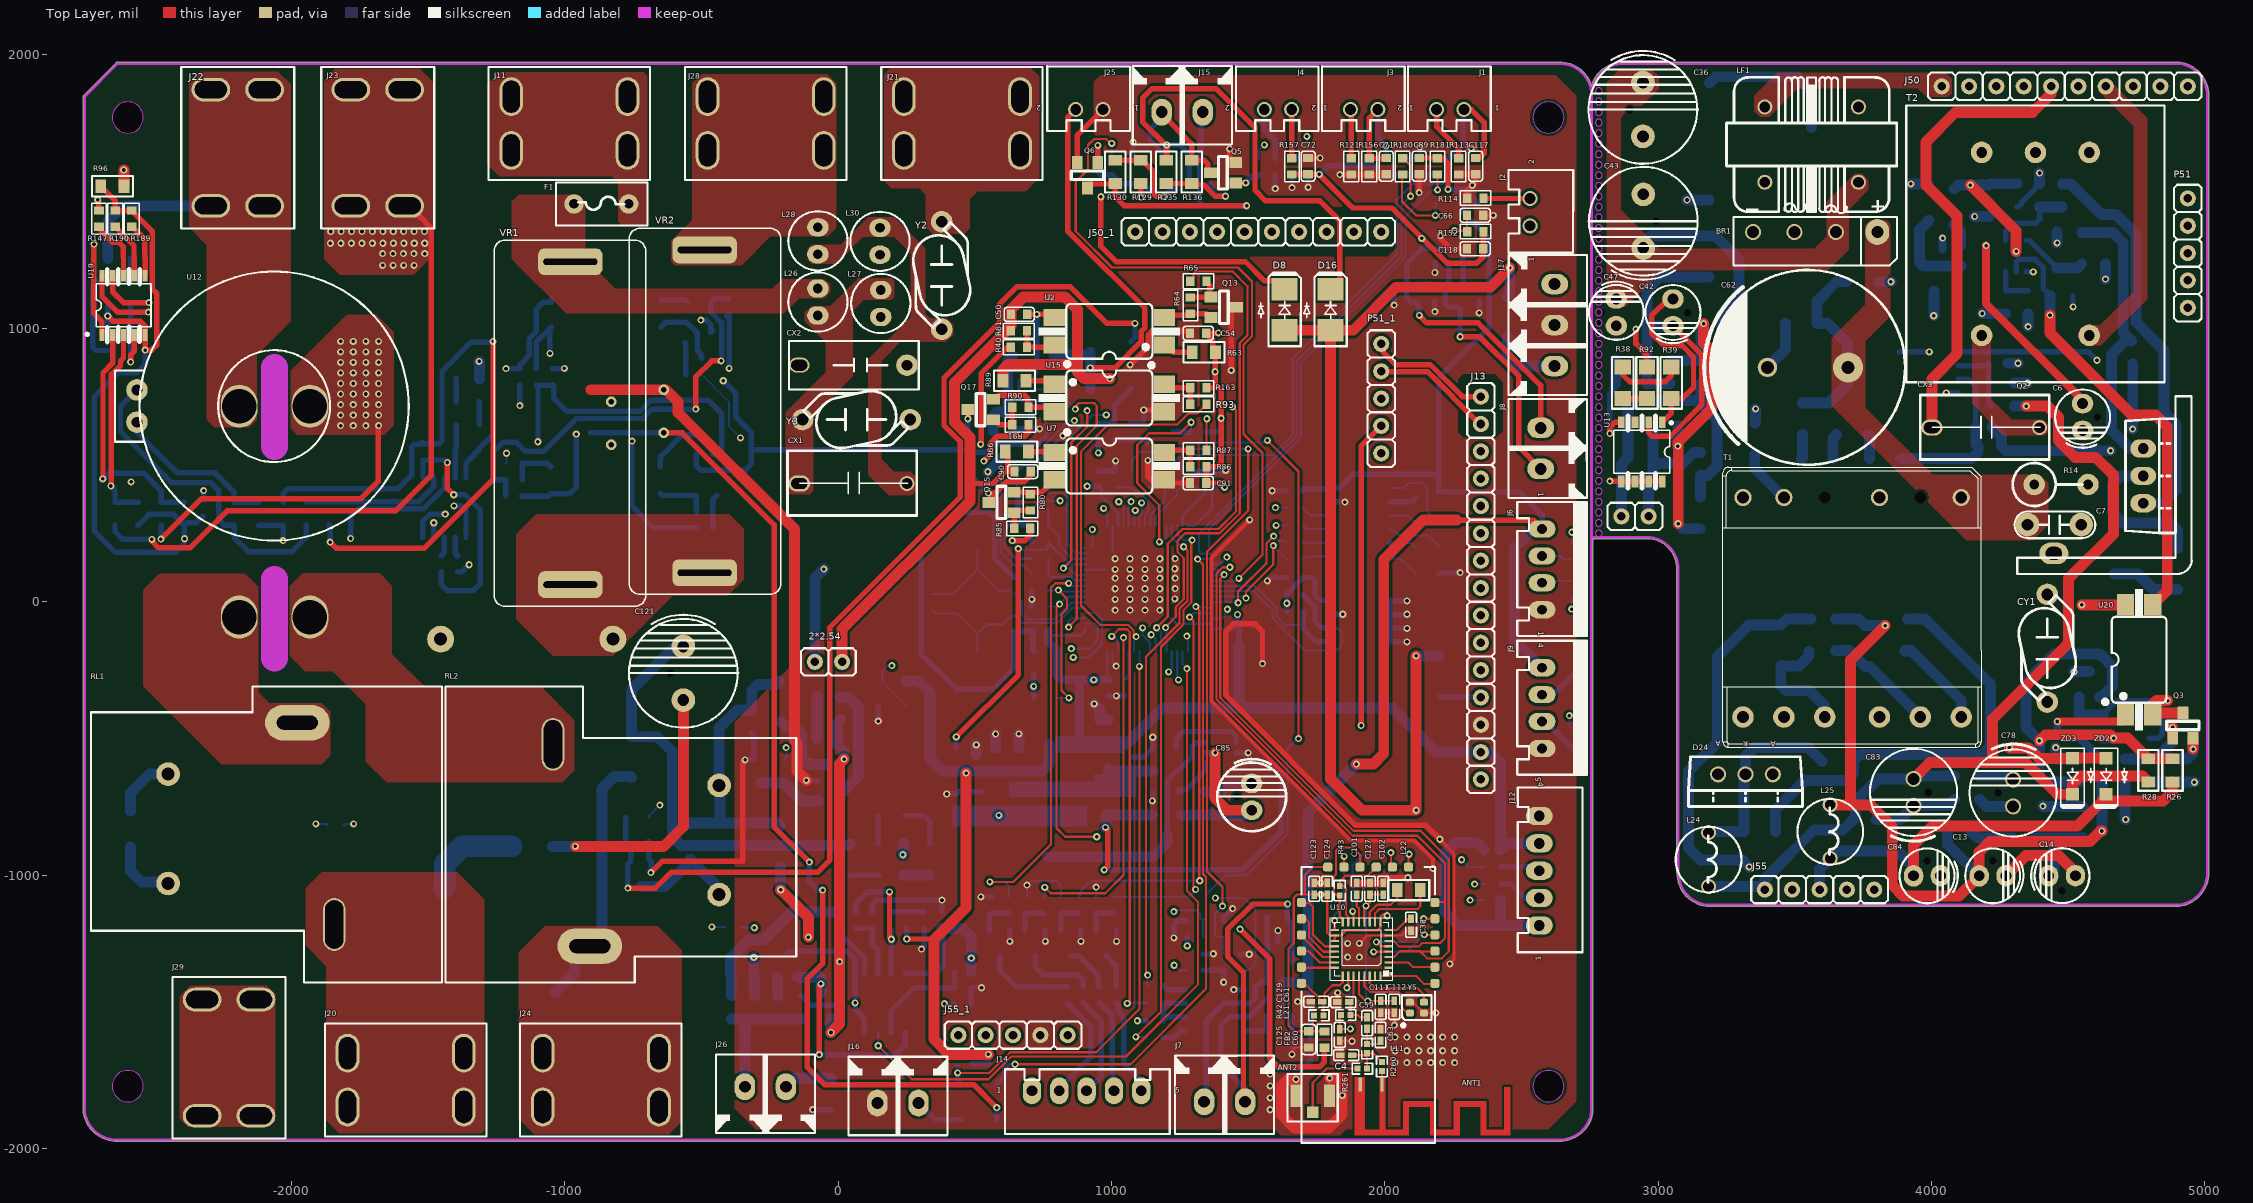
[diagram p0: Top Layer view]
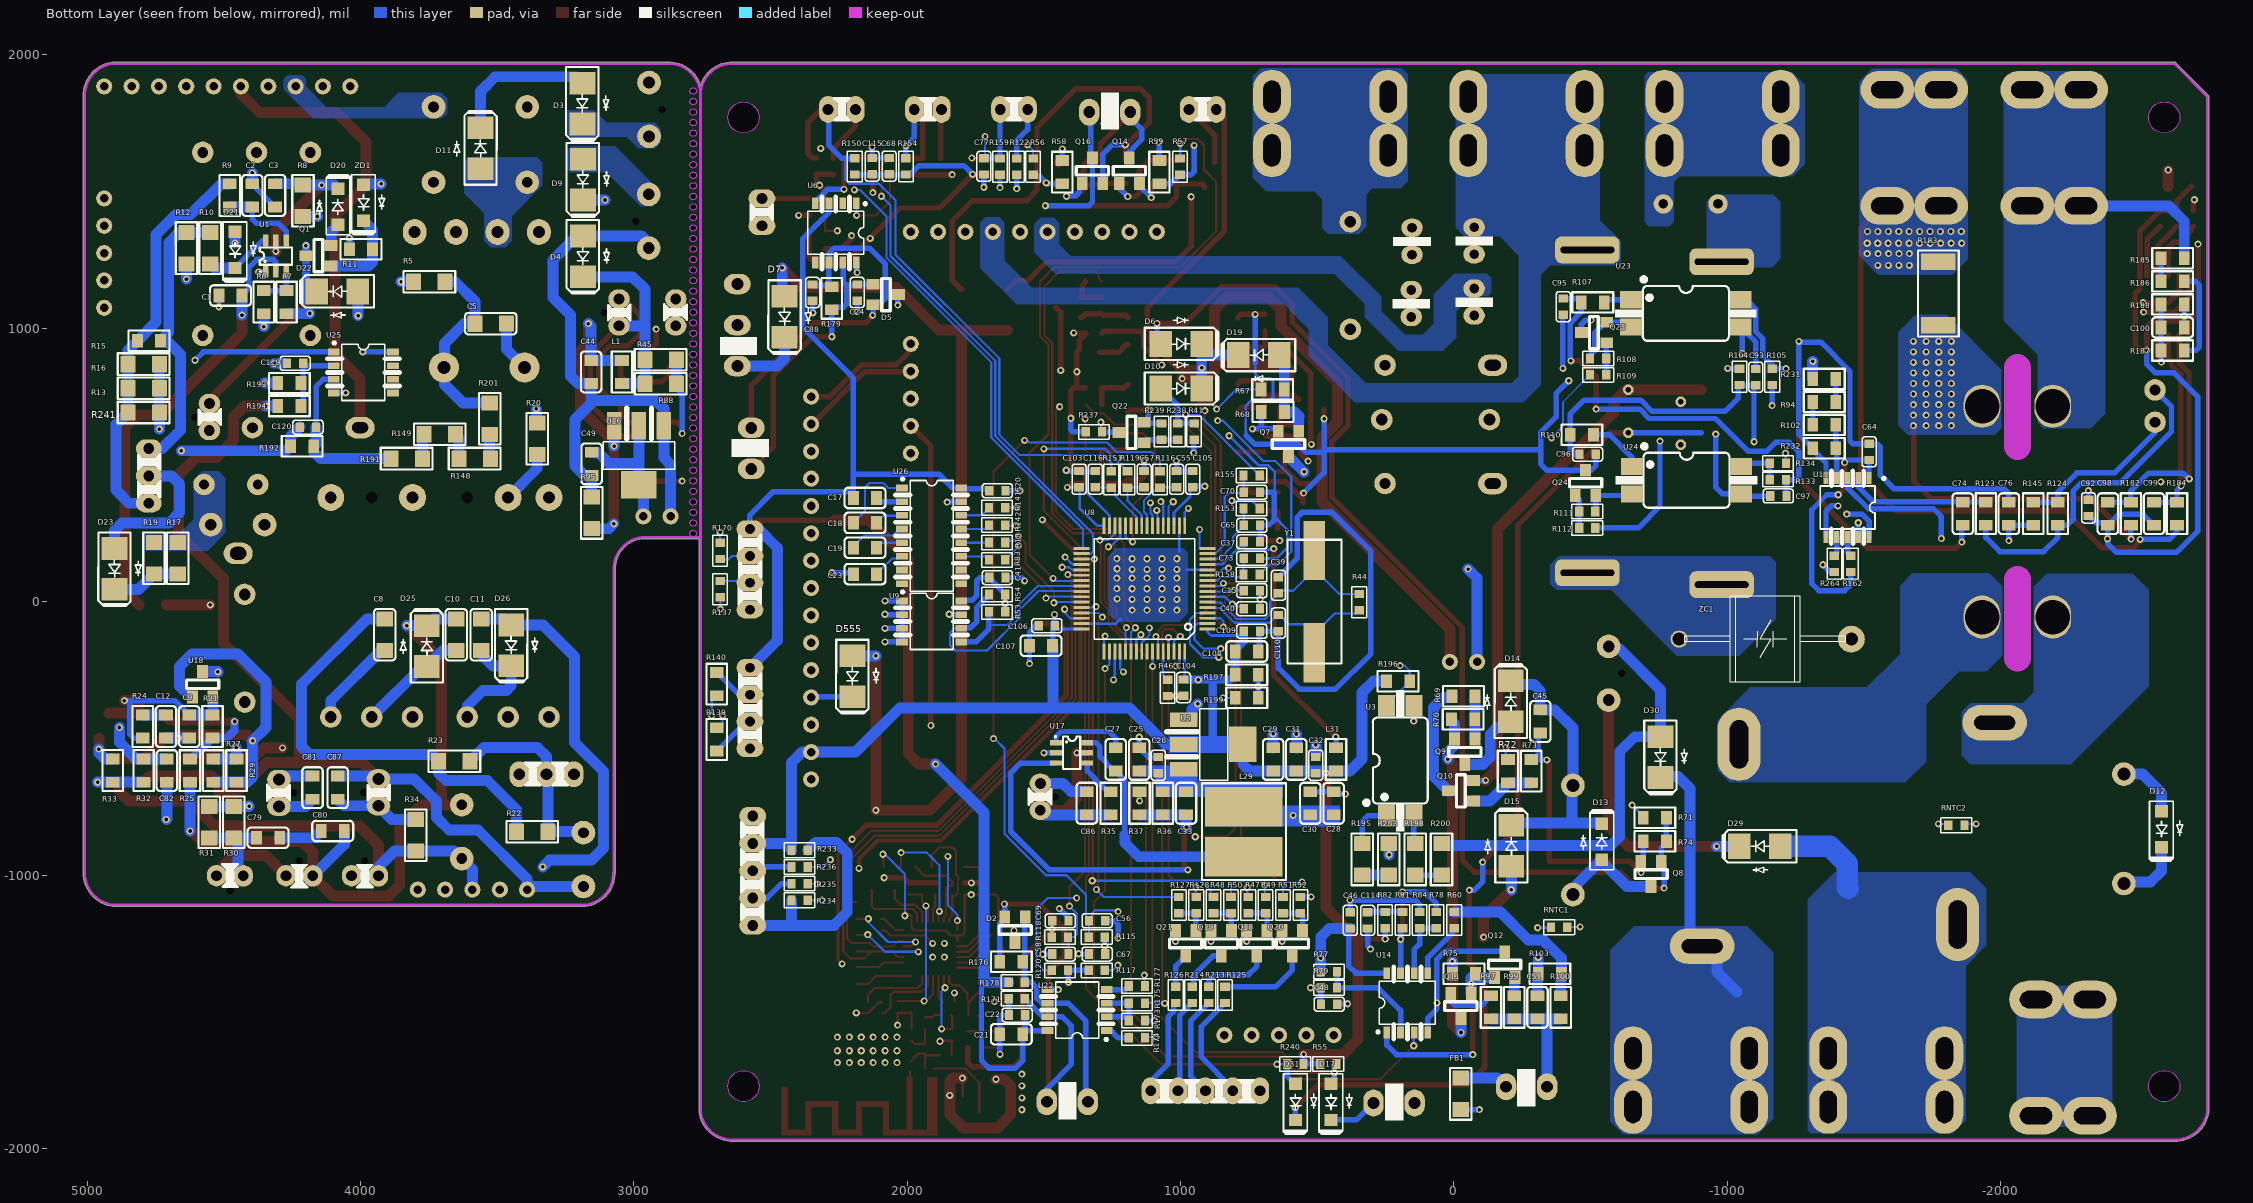
[diagram p1: Bottom Layer view, seen from below]
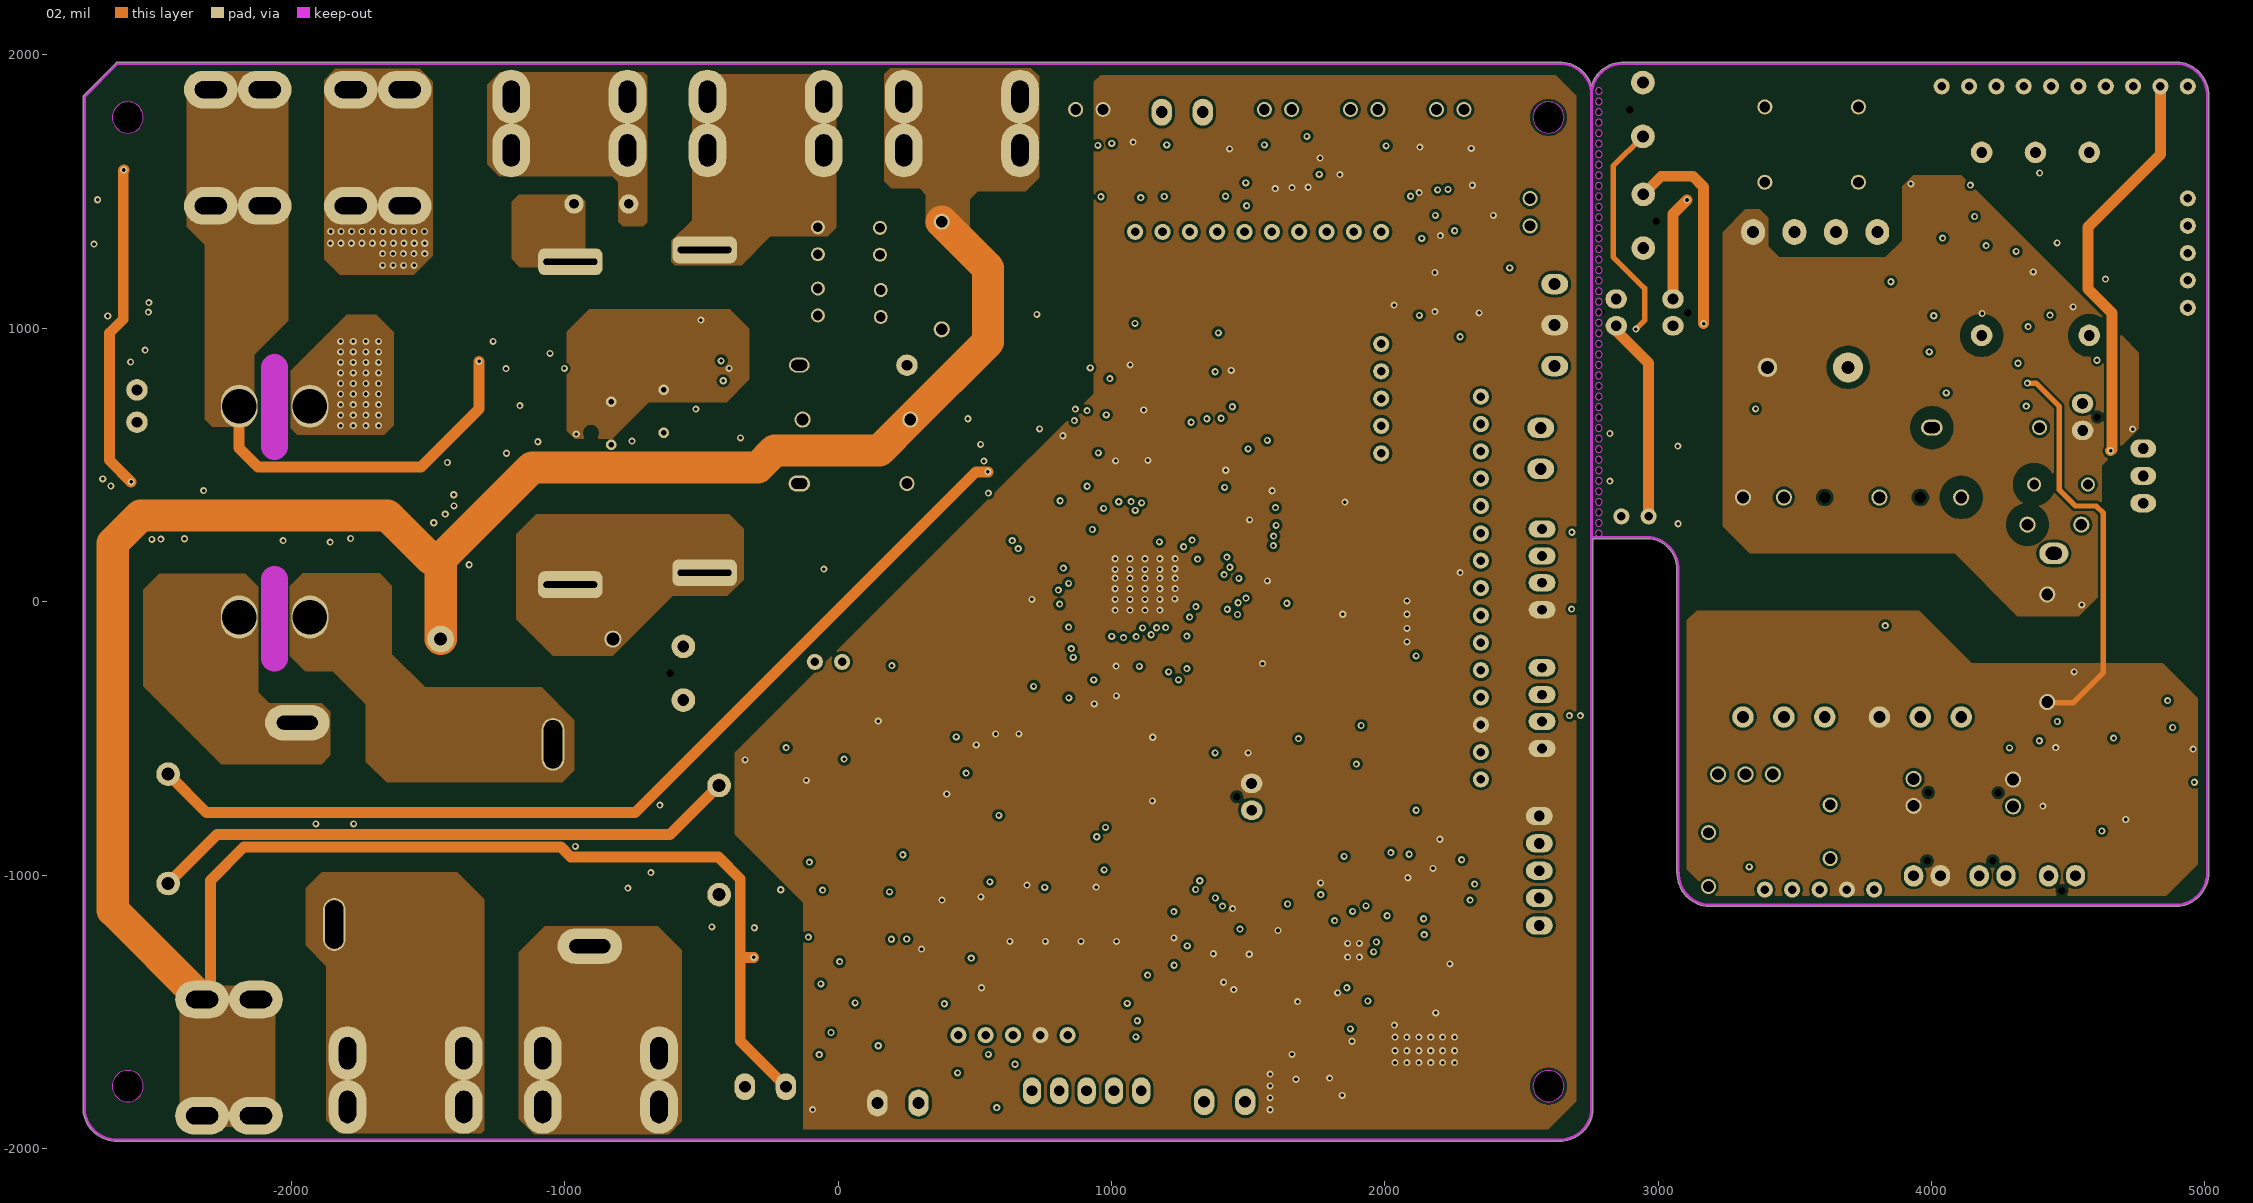
[diagram p2: 02]
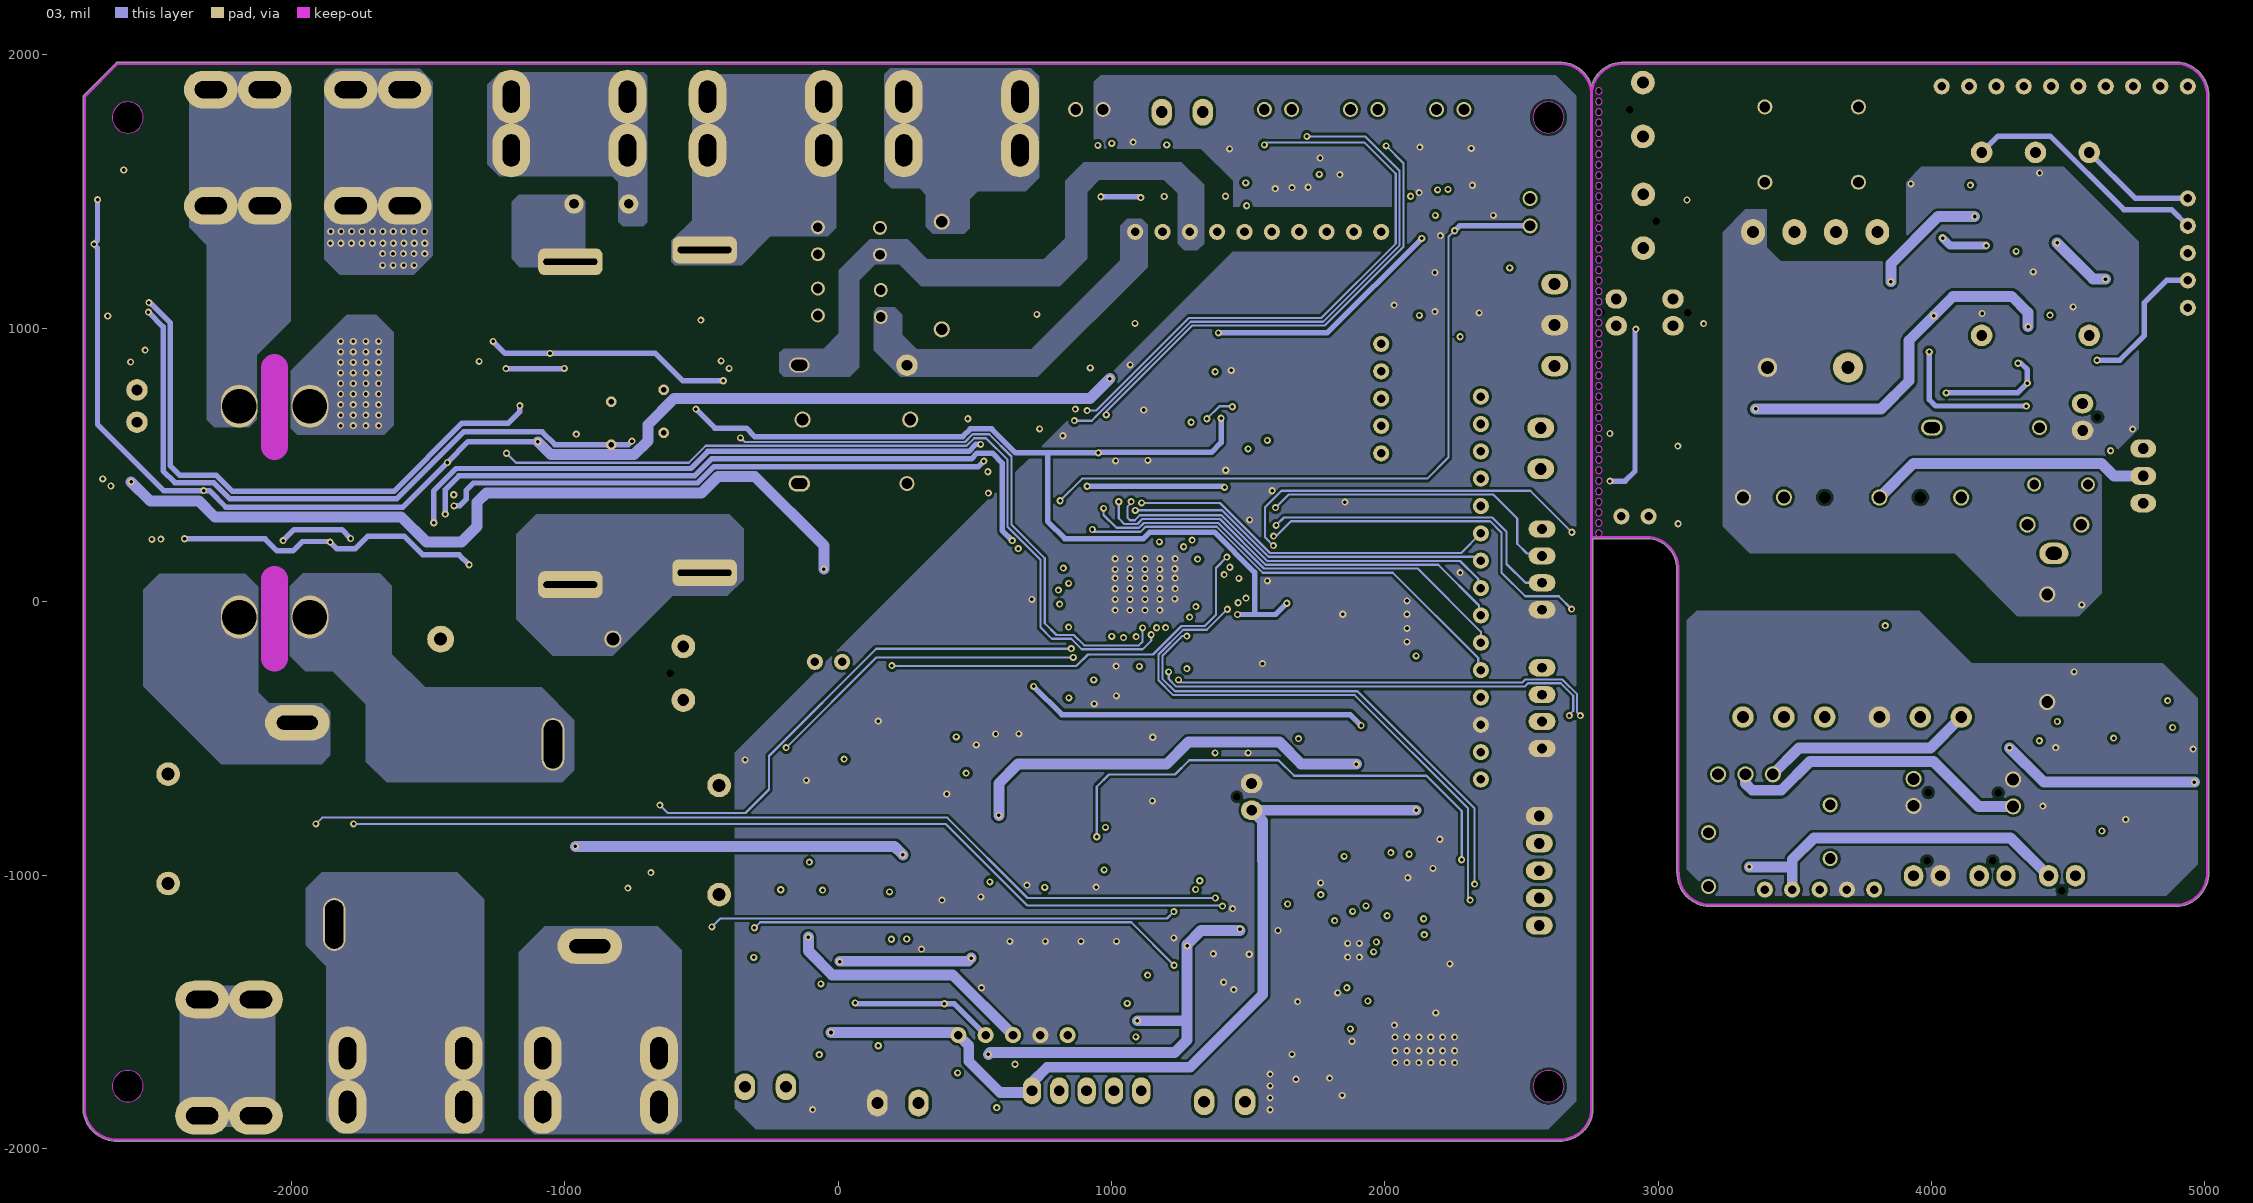
[diagram p3: 03]
# Altium PCB MISC105418.PcbDoc (part 1 of 7)
Units mil, origin at the board's own origin, x right, y up, seen from the top; angles counter-clockwise.
Board outline 7774.32 x 3947.04 mil, 4 copper layers (Top Layer, 02, 03, Bottom Layer), stack 30.635 mil thick; 459 components, 285 nets, 1258 pads, 468 vias.
Unrouted connection lines stored in the file: 23.

## Layer stack, top to bottom
Top Solder: solder mask 0.4, Solder Resist, Dk 3.5
Top Layer: signal copper 1.4
Dielectric 1: core 10, FR-4, Dk 4.2
02: signal copper 1.4173
Dielectric 6: prepreg 5, Dk 4.2
03: signal copper 1.4173
Dielectric 5: core 10, Dk 4.2
Bottom Layer: signal copper 1.4
Bottom Solder: solder mask 0.4, Solder Resist, Dk 3.5

## Board outline
-2760.88,-1866.88 ccw(c-2638.86,-1850.39) -2638.06,-1973.52 ccw(c-2637.91,-1968.5) -2637.91,-1973.52 2637.09,-1973.52 ccw(c2637.09,-1968.5) 2637.42,-1973.51 ccw(c2639.05,-1850.39) 2761.06,-1866.88 ccw(c2756.09,-1866.21) 2761.11,-1866.21 2761.11,230.49 2970.75,230.49 cw(c2955.28,118.46) 3068.37,119.45 ccw(c3073.28,118.46) 3068.27,118.46 3068.27,-990.5 ccw(c3073.28,-990.5) 3068.79,-992.72 ccw(c3191.91,-992.45) 3175.42,-1114.47 ccw(c3176.09,-1109.5) 3176.09,-1114.51 4906.09,-1114.51 ccw(c4906.09,-1109.5) 4906.77,-1114.47 ccw(c4890.28,-992.45) 5013.4,-992.45 ccw(c4890.28,-992.45) 5013.39,-990.41 ccw(c5008.37,-990.5) 5013,-988.56 5013,1847.57 ccw(c5008.37,1849.5) 5013.39,1849.42 ccw(c4890.28,1851.46) 5013.4,1851.46 ccw(c4890.28,1851.46) 4906.77,1973.47 ccw(c4906.09,1968.5) 4906.09,1973.52 ccw(c4906.09,1968.5) 4906.09,1973.52 2875.09,1973.52 ccw(c2875.09,1968.5) 2874.74,1973.51 ccw(c2872.95,1850.39) 2755.91,1888.6 ccw(c2638.86,1850.39) 2638.06,1973.52 ccw(c2637.91,1968.5) 2637.91,1973.52 -2636.53,1973.52 ccw(c-2636.53,1968.5) -2640.09,1972.03 -2759.47,1851.5 ccw(c-2755.91,1847.97) -2760.92,1847.97 -2760.92,-1866.21 ccw(c-2755.91,-1866.21)
cut-out: 2541.43,1771.16 ccw(c2598.52,1771.16) 2598.52,1714.07 ccw(c2598.52,1771.16) 2655.61,1771.16 ccw(c2598.52,1771.16) 2598.52,1828.24 ccw(c2598.52,1771.16)
cut-out: 2541.43,-1772.15 ccw(c2598.52,-1772.15) 2598.52,-1829.24 ccw(c2598.52,-1772.15) 2655.61,-1772.15 ccw(c2598.52,-1772.15) 2598.52,-1715.06 ccw(c2598.52,-1772.15)
cut-out: -2655.42,-1772.15 ccw(c-2598.33,-1772.15) -2598.33,-1829.24 ccw(c-2598.33,-1772.15) -2541.24,-1772.15 ccw(c-2598.33,-1772.15) -2598.33,-1715.06 ccw(c-2598.33,-1772.15)
cut-out: -2655.42,1771.16 ccw(c-2598.33,1771.16) -2598.33,1714.07 ccw(c-2598.33,1771.16) -2541.24,1771.16 ccw(c-2598.33,1771.16) -2598.33,1828.24 ccw(c-2598.33,1771.16)
cut-out: 2782.47,1879.96 ccw(c2782.47,1867.88) 2770.39,1867.88 ccw(c2782.47,1867.88) 2782.47,1855.79 ccw(c2782.47,1867.88) 2794.55,1867.88 ccw(c2782.47,1867.88)
cut-out: 2782.47,1841.42 ccw(c2782.47,1829.34) 2770.39,1829.34 ccw(c2782.47,1829.34) 2782.47,1817.26 ccw(c2782.47,1829.34) 2794.55,1829.34 ccw(c2782.47,1829.34)
cut-out: 2782.47,1802.89 ccw(c2782.47,1790.8) 2770.39,1790.8 ccw(c2782.47,1790.8) 2782.47,1778.72 ccw(c2782.47,1790.8) 2794.55,1790.8 ccw(c2782.47,1790.8)
cut-out: 2782.47,1764.35 ccw(c2782.47,1752.27) 2770.39,1752.27 ccw(c2782.47,1752.27) 2782.47,1740.19 ccw(c2782.47,1752.27) 2794.55,1752.27 ccw(c2782.47,1752.27)
cut-out: 2782.47,1725.81 ccw(c2782.47,1713.73) 2770.39,1713.73 ccw(c2782.47,1713.73) 2782.47,1701.65 ccw(c2782.47,1713.73) 2794.55,1713.73 ccw(c2782.47,1713.73)
cut-out: 2782.47,1687.28 ccw(c2782.47,1675.19) 2770.39,1675.19 ccw(c2782.47,1675.19) 2782.47,1663.11 ccw(c2782.47,1675.19) 2794.55,1675.19 ccw(c2782.47,1675.19)
cut-out: 2782.47,1648.74 ccw(c2782.47,1636.66) 2770.39,1636.66 ccw(c2782.47,1636.66) 2782.47,1624.58 ccw(c2782.47,1636.66) 2794.55,1636.66 ccw(c2782.47,1636.66)
cut-out: 2782.47,1610.2 ccw(c2782.47,1598.12) 2770.39,1598.12 ccw(c2782.47,1598.12) 2782.47,1586.04 ccw(c2782.47,1598.12) 2794.55,1598.12 ccw(c2782.47,1598.12)
cut-out: 2782.47,1571.67 ccw(c2782.47,1559.59) 2770.39,1559.59 ccw(c2782.47,1559.59) 2782.47,1547.5 ccw(c2782.47,1559.59) 2794.55,1559.59 ccw(c2782.47,1559.59)
cut-out: 2782.47,1533.13 ccw(c2782.47,1521.05) 2770.39,1521.05 ccw(c2782.47,1521.05) 2782.47,1508.97 ccw(c2782.47,1521.05) 2794.55,1521.05 ccw(c2782.47,1521.05)
cut-out: 2782.47,1494.59 ccw(c2782.47,1482.51) 2770.39,1482.51 ccw(c2782.47,1482.51) 2782.47,1470.43 ccw(c2782.47,1482.51) 2794.55,1482.51 ccw(c2782.47,1482.51)
cut-out: 2782.47,1456.06 ccw(c2782.47,1443.98) 2770.39,1443.98 ccw(c2782.47,1443.98) 2782.47,1431.89 ccw(c2782.47,1443.98) 2794.55,1443.98 ccw(c2782.47,1443.98)
cut-out: 2782.47,1417.52 ccw(c2782.47,1405.44) 2770.39,1405.44 ccw(c2782.47,1405.44) 2782.47,1393.36 ccw(c2782.47,1405.44) 2794.55,1405.44 ccw(c2782.47,1405.44)
cut-out: 2782.47,1378.99 ccw(c2782.47,1366.9) 2770.39,1366.9 ccw(c2782.47,1366.9) 2782.47,1354.82 ccw(c2782.47,1366.9) 2794.55,1366.9 ccw(c2782.47,1366.9)
cut-out: 2782.47,1340.45 ccw(c2782.47,1328.37) 2770.39,1328.37 ccw(c2782.47,1328.37) 2782.47,1316.28 ccw(c2782.47,1328.37) 2794.55,1328.37 ccw(c2782.47,1328.37)
cut-out: 2782.47,1301.91 ccw(c2782.47,1289.83) 2770.39,1289.83 ccw(c2782.47,1289.83) 2782.47,1277.75 ccw(c2782.47,1289.83) 2794.55,1289.83 ccw(c2782.47,1289.83)
cut-out: 2782.47,1263.38 ccw(c2782.47,1251.29) 2770.39,1251.29 ccw(c2782.47,1251.29) 2782.47,1239.21 ccw(c2782.47,1251.29) 2794.55,1251.29 ccw(c2782.47,1251.29)
cut-out: 2782.47,1224.84 ccw(c2782.47,1212.76) 2770.39,1212.76 ccw(c2782.47,1212.76) 2782.47,1200.67 ccw(c2782.47,1212.76) 2794.55,1212.76 ccw(c2782.47,1212.76)
cut-out: 2782.47,1200.67 ccw(c2782.47,1212.76) 2794.55,1212.76 ccw(c2782.47,1212.76) 2782.47,1224.84 ccw(c2782.47,1212.76) 2770.39,1212.76 ccw(c2782.47,1212.76)
cut-out: 2782.47,1162.14 ccw(c2782.47,1174.22) 2794.55,1174.22 ccw(c2782.47,1174.22) 2782.47,1186.3 ccw(c2782.47,1174.22) 2770.39,1174.22 ccw(c2782.47,1174.22)
cut-out: 2782.47,1123.6 ccw(c2782.47,1135.68) 2794.55,1135.68 ccw(c2782.47,1135.68) 2782.47,1147.77 ccw(c2782.47,1135.68) 2770.39,1135.68 ccw(c2782.47,1135.68)
cut-out: 2782.47,1085.06 ccw(c2782.47,1097.15) 2794.55,1097.15 ccw(c2782.47,1097.15) 2782.47,1109.23 ccw(c2782.47,1097.15) 2770.39,1097.15 ccw(c2782.47,1097.15)
cut-out: 2782.47,1046.53 ccw(c2782.47,1058.61) 2794.55,1058.61 ccw(c2782.47,1058.61) 2782.47,1070.69 ccw(c2782.47,1058.61) 2770.39,1058.61 ccw(c2782.47,1058.61)
cut-out: 2782.47,1007.99 ccw(c2782.47,1020.07) 2794.55,1020.07 ccw(c2782.47,1020.07) 2782.47,1032.16 ccw(c2782.47,1020.07) 2770.39,1020.07 ccw(c2782.47,1020.07)
cut-out: 2782.47,969.45 ccw(c2782.47,981.54) 2794.55,981.54 ccw(c2782.47,981.54) 2782.47,993.62 ccw(c2782.47,981.54) 2770.39,981.54 ccw(c2782.47,981.54)
cut-out: 2782.47,930.92 ccw(c2782.47,943) 2794.55,943 ccw(c2782.47,943) 2782.47,955.08 ccw(c2782.47,943) 2770.39,943 ccw(c2782.47,943)
cut-out: 2782.47,892.38 ccw(c2782.47,904.46) 2794.55,904.46 ccw(c2782.47,904.46) 2782.47,916.55 ccw(c2782.47,904.46) 2770.39,904.46 ccw(c2782.47,904.46)
cut-out: 2782.47,853.84 ccw(c2782.47,865.93) 2794.55,865.93 ccw(c2782.47,865.93) 2782.47,878.01 ccw(c2782.47,865.93) 2770.39,865.93 ccw(c2782.47,865.93)
cut-out: 2782.47,815.31 ccw(c2782.47,827.39) 2794.55,827.39 ccw(c2782.47,827.39) 2782.47,839.47 ccw(c2782.47,827.39) 2770.39,827.39 ccw(c2782.47,827.39)
cut-out: 2782.47,776.77 ccw(c2782.47,788.85) 2794.55,788.85 ccw(c2782.47,788.85) 2782.47,800.94 ccw(c2782.47,788.85) 2770.39,788.85 ccw(c2782.47,788.85)
cut-out: 2782.47,738.23 ccw(c2782.47,750.32) 2794.55,750.32 ccw(c2782.47,750.32) 2782.47,762.4 ccw(c2782.47,750.32) 2770.39,750.32 ccw(c2782.47,750.32)
cut-out: 2782.47,699.7 ccw(c2782.47,711.78) 2794.55,711.78 ccw(c2782.47,711.78) 2782.47,723.86 ccw(c2782.47,711.78) 2770.39,711.78 ccw(c2782.47,711.78)
cut-out: 2782.47,661.16 ccw(c2782.47,673.24) 2794.55,673.24 ccw(c2782.47,673.24) 2782.47,685.33 ccw(c2782.47,673.24) 2770.39,673.24 ccw(c2782.47,673.24)
cut-out: 2782.47,622.62 ccw(c2782.47,634.71) 2794.55,634.71 ccw(c2782.47,634.71) 2782.47,646.79 ccw(c2782.47,634.71) 2770.39,634.71 ccw(c2782.47,634.71)
cut-out: 2782.47,584.09 ccw(c2782.47,596.17) 2794.55,596.17 ccw(c2782.47,596.17) 2782.47,608.25 ccw(c2782.47,596.17) 2770.39,596.17 ccw(c2782.47,596.17)
cut-out: 2782.47,545.55 ccw(c2782.47,557.63) 2794.55,557.63 ccw(c2782.47,557.63) 2782.47,569.72 ccw(c2782.47,557.63) 2770.39,557.63 ccw(c2782.47,557.63)
cut-out: 2782.47,507.01 ccw(c2782.47,519.1) 2794.55,519.1 ccw(c2782.47,519.1) 2782.47,531.18 ccw(c2782.47,519.1) 2770.39,519.1 ccw(c2782.47,519.1)
cut-out: 2782.47,429.94 ccw(c2782.47,442.02) 2794.55,442.02 ccw(c2782.47,442.02) 2782.47,454.11 ccw(c2782.47,442.02) 2770.39,442.02 ccw(c2782.47,442.02)
cut-out: 2782.47,622.62 ccw(c2782.47,634.71) 2794.55,634.71 ccw(c2782.47,634.71) 2782.47,646.79 ccw(c2782.47,634.71) 2770.39,634.71 ccw(c2782.47,634.71)
cut-out: 2782.47,584.09 ccw(c2782.47,596.17) 2794.55,596.17 ccw(c2782.47,596.17) 2782.47,608.25 ccw(c2782.47,596.17) 2770.39,596.17 ccw(c2782.47,596.17)
cut-out: 2782.47,545.55 ccw(c2782.47,557.63) 2794.55,557.63 ccw(c2782.47,557.63) 2782.47,569.72 ccw(c2782.47,557.63) 2770.39,557.63 ccw(c2782.47,557.63)
cut-out: 2782.47,507.01 ccw(c2782.47,519.1) 2794.55,519.1 ccw(c2782.47,519.1) 2782.47,531.18 ccw(c2782.47,519.1) 2770.39,519.1 ccw(c2782.47,519.1)
cut-out: 2782.47,468.48 ccw(c2782.47,480.56) 2794.55,480.56 ccw(c2782.47,480.56) 2782.47,492.64 ccw(c2782.47,480.56) 2770.39,480.56 ccw(c2782.47,480.56)
cut-out: 2782.47,391.4 ccw(c2782.47,403.49) 2794.55,403.49 ccw(c2782.47,403.49) 2782.47,415.57 ccw(c2782.47,403.49) 2770.39,403.49 ccw(c2782.47,403.49)
cut-out: 2782.47,352.87 ccw(c2782.47,364.95) 2794.55,364.95 ccw(c2782.47,364.95) 2782.47,377.03 ccw(c2782.47,364.95) 2770.39,364.95 ccw(c2782.47,364.95)
cut-out: 2782.47,314.33 ccw(c2782.47,326.41) 2794.55,326.41 ccw(c2782.47,326.41) 2782.47,338.5 ccw(c2782.47,326.41) 2770.39,326.41 ccw(c2782.47,326.41)
cut-out: 2782.47,275.79 ccw(c2782.47,287.88) 2794.55,287.88 ccw(c2782.47,287.88) 2782.47,299.96 ccw(c2782.47,287.88) 2770.39,287.88 ccw(c2782.47,287.88)
cut-out: 2782.47,237.26 ccw(c2782.47,249.34) 2794.55,249.34 ccw(c2782.47,249.34) 2782.47,261.42 ccw(c2782.47,249.34) 2770.39,249.34 ccw(c2782.47,249.34)

## Design rules (kind name [scope] priority, off if disabled: settings)
Clearance [All] p1: gap=6 except(10: Arc-Fill Arc-Poly Arc-Region Track-Fill Track-Poly Track-Region SMDPad-Fill SMDPad-Poly SMDPad-Region THPad-Fill THPad-Poly THPad-Region Via-Fill Via-Poly Via-Region Fill-Fill Fill-Poly Fill-Region Poly-Poly Poly-Region Region-Region)
PlaneConnect [All] p1: planeconnectstyle=NoConnect reliefexpansion=20 reliefentries=4 reliefconductorwidth=10 reliefairgap=10
PolygonConnect [All] p1: connectstyle=Direct reliefconductorwidth=10 reliefentries=4 polygonreliefangle="90 Angle" airgapwidth=10
RoutingVias [All] p1: holewidth=13 width=26 viastyle="Through Hole" minholewidth=1 minwidth=1 maxholewidth=50 maxwidth=50
SolderMaskExpansion [All] p1: expansion=4
Width [All] p1: maxlimit=500 minlimit=6 preferedwidth=8
29 further rules are at their usual default settings.

## Classes and differential pairs
component class RELAY_V0.1: C15 C45 C46 C48 C51 C114 C119 C120 C121 D6 D10 D12 D13 D14 D15 D19 D29 D30 FB1 J20 J21 J22 J23 J24 J25 J26 J29 Q7 Q8 Q9 Q10 Q11 Q12 R60 R67 R68 R69 R70 R71 R72 R73 R74 R75 R77 R78 R79 R81 R82 R84 R97 R99 R100 R103 R148 R149 R183 R191 R192 R193 R194 R195 R196 R197 R198 R199 R200 R201 R263 RL1 RL2 U3 U14 U25
component class POWER_V0.1: BR1 C1 C2 C3 C5 C6 C7 C8 C9 C10 C11 C12 C13 C14 C25 C26 C27 C28 C29 C30 C31 C32 C33 C36 C42 C43 C44 C47 C49 C62 C78 C79 C80 C81 C82 C83 C84 C85 C86 C87 CX1 CX2 CX3 CY1 D3 D4 D7 D9 D11 D20 D21 D22 D23 D24 D25 D26 F1 J11 J17 J28 J50 J55 L1 L24 L25 L26 L27 L28 L29 L30 L31 LF1 P51 Q1 Q2 Q3 R5 R6 R7 R8 R9 R10 R11 R12 R13 R14 R15 R16 R17 R19 R20 R21 R22 R23 R24 R25 R26 R27 R28 R29 R30 R31 R32 R33 R34 R35 R36 R37 R38 R39 R45 R88 R92 R95 R241 T1 T2 U1 U5 U13 U16 U17 U18 U20 VR1 VR2 Y2 Y3 ZC1 ZD1 ZD2 ZD3
component class "MCU Controller for 7KW_V0.1": C37 C39 C40 C41 C103 C104 C105 C106 C107 C108 C109 C110 D17 D31 D555 J12 J13 J14 J16 Q18 Q19 Q20 Q21 Q22 R41 R44 R46 R47 R48 R49 R50 R51 R52 R53 R54 R55 R125 R126 R127 R128 R213 R214 R233 R234 R235 R236 R237 R238 R239 R240 U8 U9 Y1
component class ElectricLeakage-Check_V0.1: C50 C54 C64 C74 C76 C90 C91 C92 C93 C95 C96 C97 C98 C99 C100 Q13 Q15 Q17 Q23 Q24 R40 R61 R63 R64 R65 R66 R80 R85 R86 R87 R89 R90 R91 R93 R94 R96 R102 R104 R105 R107 R108 R109 R110 R111 R112 R123 R124 R133 R134 R145 R147 R162 R163 R182 R184 R185 R186 R187 R188 R189 R190 R231 R232 R264 U2 U7 U11 U12 U15 U19 U23 U24
component class Communication_V0.1: C17 C18 C19 C20 C21 C22 C23 C24 C88 C89 D2 D5 J6 J7 J8 J9 R18 R83 R137 R139 R140 R141 R142 R170 R171 R173 R174 R175 R176 R177 R178 R179 R180 R181 U6 U22 U26
component class BLE_V0.1: ANT1 ANT2 C4 C38 C59 C60 C61 C63 C101 C102 C111 C112 C123 C124 C125 C127 C129 FB2 L11 L21 L22 R42 R43 R260 R261 U10 Y5
component class ADC_V0.1: C55 C56 C57 C58 C65 C66 C67 C68 C69 C70 C71 C72 C73 C77 C115 C116 C117 C118 D8 D16 J1 J2 J3 J4 J15 Q5 Q6 Q14 Q16 R56 R57 R58 R59 R113 R114 R115 R116 R117 R118 R119 R120 R121 R122 R129 R130 R135 R136 R150 R151 R152 R153 R154 R155 R156 R157 R158 R159 RNTC1 RNTC2

## Components (designator, comment, footprint, x,y, rotation, side; value= is the part's Value field where it differs from the comment)
2*2.54 "Comment" p2-2.54 14.72,-220.24 r180 top
ANT1 "PCB onboard antenna" ATN 1949.33,-1767 r0 top
ANT2 "ANT_SMA" ATN-1 1736,-1807 r90 top
BR1 "KBJ2J" BD15.22X4.5(KBP206）RS-2 3574.21,1352 r180 top
C1 "1nF" C0805-T 4475,1120 r0 bottom
C2 "100pF" C0805-T 4395.09,1486.02 r90 bottom
C3 "0.1uF" C0805-T 4312.09,1486.02 r270 bottom
C4 "0.5pF/50V" C0402-T 1859.09,-1659.03 r180 top
C5 "10nF/1KV" C1206-T 3523,1017 r180 bottom
C6 "22uF/50V" CE5-P2.5MM-AI-DS 4552.29,675.49 r270 top
C7 "222/1KV" CC7.5-P5.0MM-AI-2.5-DS 4449.09,281.5 r180 top
C8 "102/1KV" C1206-T 3911,-120.96 r90 bottom
C9 "0.1uF" C0805-T 4626.09,-456.82 r270 bottom
C10 "n.c" C1206-T 3649.09,-120.96 r90 bottom
C11 "n.c" C1206-T 3558.09,-120.96 r90 bottom
C12 "N.C" C0805-T 4711.09,-456.82 r270 bottom
C13 "100uF/16V" CE5-P2.5MM-AI-DS 4223.09,-1002.69 r0 top
C14 "100uF/16V" CE5-P2.5MM-AI-DS 4477.09,-1002.68 r180 top
C15 "0.1uF/50V" C0603-T 738.8,40.36 r180 bottom
C17 "1uF/50V" CAP/0805 2154,379 r180 bottom
C18 "1uF/50V" CAP/0805 2154,288.12 r0 bottom
C19 "1uF/50V" CAP/0805 2154,197.52 r0 bottom
C20 "0.1uF/50V" CAP/0603 1669.91,405.7 r180 bottom
C21 "10uF/10V" C0805-T 1618.98,-1582.14 r0 bottom
C22 "0.1uF/50V" C0603-T 1597.86,-1512.14 r0 bottom
C23 "1uF/50V" CAP/0805 2154.09,100.7 r180 bottom
C24 "15pF/50V" C0603-T 2183,1130.77 r90 bottom
C25 "10uF/10V" C0805-T 1151.09,-576.97 r90 bottom
C26 "0.1uF/50V" C0603-T 1081.09,-598.09 r90 bottom
C27 "0.1uF" C0805-T 1237.09,-576.97 r270 bottom
C28 "10uF/10V" C0805-T 439.9,-737.5 r90 bottom
C29 "10uF/10V" C0805-T 661.09,-576.97 r90 bottom
C30 "10uF/10V" C0805-T 524.9,-737.5 r90 bottom
C31 "10uF/10V" C0805-T 576.09,-576.97 r90 bottom
C32 "0.1uF/50V" C0603-T 505.11,-598.09 r90 bottom
C33 "47pF" C0805-T 980.08,-737.5 r270 bottom
C36 "10uF/400V" CE10-P5.0MM-AI 2945.37,1800.82 r90 top
C37 "0.1uF/50V" C0603-T 738.8,218.65 r0 bottom
C38 "1uF/50V" C0402-T 2096,-1182 r90 top
C39 "20pF/50V" C0603-T 642,60 r270 bottom
C40 "0.1uF/50V" C0603-T 738.8,-26.07 r180 bottom
C41 "0.1uF/50V" C0603-T 1669.91,88.29 r0 bottom
C42 "10uF/50V" CE5-P2.5MM-AI 3054,1058 r270 top
C43 "100uF/25V" CE10-P5.0MM-AI 2943.98,1391.21 r270 top
C44 "1uF/25V" C0805-T 3156,840.12 r90 bottom
C45 "0.1uF/50V" C0805-T -316,-438.06 r270 bottom
C46 "0.1uF/50V" C0603-T 378.89,-1165.89 r270 bottom
C47 "100uF/16V" CE5-P2.5MM-AI 2846.39,1058 r90 top
C48 "0.1uF/50V" C0603-T 456.03,-1472.5 r0 bottom
C49 "1uF/25V/0805" C0805-T 3154,504 r90 bottom
C50 "0.1uF/50V" C0603-T 662.34,1050.81 r180 top
C51 "NC" C0805-T -305.91,-1483.82 r90 bottom
C54 "0.1uF/50V" C0603-T 1316.93,981.91 r180 top
C55 "0.1uF/50V" C0603-T 1014.43,448 r90 bottom
C56 "0.1uF/50V" C0603-T 1305.17,-1167.62 r0 bottom
C57 "0.1uF/50V" C0603-T 1133.29,448 r90 bottom
C58 "0.1uF/50V" C0603-T 1439.72,-1289.07 r180 bottom
C59 "220pF/50V" C0402-T 1935.09,-1541.57 r90 top
C60 "18pF/50V" C0402-T 1835.09,-1585.03 r90 top
C61 "2.7pF/50V" C0402-T 1848.09,-1465.03 r0 top
C62 "47uF/400V" CE18 3547,857 r180 top
C63 "2pF/50V" C0402-T 1984.09,-1585.03 r270 top
C64 "0.1uF/50V" C0603-T -1519,548 r90 bottom
C65 "0.1uF/50V" C0603-T 738.8,279.08 r180 bottom
C66 "0.1uF/50V" C0603-T 2330.19,1413.53 r0 top
C67 "0.1uF/50V" C0603-T 1305.17,-1289.07 r180 bottom
C68 "0.1uF/50V" C0603-T 2065.9,1593.18 r270 bottom
C69 "0.1uF/50V" C0603-T 1439.72,-1167.62 r0 bottom
C70 "0.1uF/50V" C0603-T 738.8,399.93 r180 bottom
C71 "0.1uF/50V" C0603-T 2005,1593.18 r270 top
C72 "0.1uF/50V" C0603-T 1719,1593.14 r270 top
C73 "0.1uF/50V" C0603-T 738.8,158.22 r180 bottom
C74 "33nF" C0805-T -1861.91,321.64 r90 bottom
C76 "33nF" C0805-T -2030.15,321.64 r270 bottom
C77 "0.1uF/50V" C0603-T 1719.09,1592.14 r270 bottom
C78 "680uF/25V" CE8-P2.5MM-AI-DS 4298.98,-699.71 r90 top
C79 "0.1uF" C0805-T 4337.7,-863.75 r180 bottom
C80 "0.1uF" C0805-T 4101.09,-839.18 r180 bottom
C81 "0.1uF" C0805-T 4175.09,-680.5 r270 bottom
C82 "10nF" C0805-T 4708.09,-618.17 r270 bottom
C83 "470uF/25V" CE8-P2.5MM-AI-DS 3933.09,-697.5 r270 top
C84 "100uF/16V" CE5-P2.5MM-AI-DS 3983.08,-1002.69 r0 top
C85 "22u/50V" CE6.3-P2.5MM-AI-DS 1512.8,-713.98 r90 top
C86 "0.1uF" C0805-T 1343.09,-737.5 r270 bottom
C87 "0.1uF" C0805-T 4083.09,-680.5 r90 bottom
C88 "15pF/50V" C0603-T 2346.09,1130.77 r270 bottom
C89 "15pF/50V" C0603-T 2126,1593.18 r270 top
C90 "0.1uF/50V" C0603-T 674.8,476 r180 top
C91 "0.1uF/50V" C0603-T 1316.93,434 r0 top
C92 "0.1uF/50V" C0603-T -2321.4,342.76 r270 bottom
C93 "0.1uF/50V" C0603-T -1104.5,821.3 r270 bottom
C95 "0.1uF/50V" C0603-T -400,1079 r270 bottom
C96 "0.1uF/50V" C0603-T -489.03,539.5 r0 bottom
C97 "0.1uF/50V" C0603-T -1186.7,386.5 r180 bottom
C98 "33nF" C0805-T -2392.18,321.64 r270 bottom
C99 "33nF" C0805-T -2560.91,321.64 r90 bottom
C100 "33nF" C0805-T -2629.23,1002.7 r180 bottom
C101 "1uF" C0402-T 1897,-1050.03 r90 top
C102 "2.2uF" C0402-T 1993.76,-1050.03 r270 top
C103 "0.1uF/50V" C0603-T 1371,448 r90 bottom
C104 "0.1uF/50V" C0603-T 989,-314.28 r270 bottom
C105 "0.1uF/50V" C0603-T 955,448 r90 bottom
C106 "0.1uF/50V" C0603-T 1489,-88 r0 bottom
C107 "10uF/10V" C0805-T 1510.12,-161 r0 bottom
C108 "10uF/10V" C0805-T 757.68,-182.5 r180 bottom
C109 "0.1uF/50V" C0603-T 738.8,-108.5 r0 bottom
C110 "20pF/50V" C0603-T 642,-78.28 r270 bottom
C111 "0.1uF" C0402-T 1984.76,-1482.25 r270 top
C112 "1uF" C0402-T 2034.17,-1482.25 r270 top
C114 "1nF/50V" C0603-T 315.76,-1165.89 r270 bottom
C115 "0.1uF/50V" C0603-T 2128.17,1593.18 r270 bottom
C116 "0.1uF/50V" C0603-T 1311.57,448 r90 bottom
C117 "0.1uF/50V" C0603-T 2332,1593.18 r90 top
C118 "0.1uF/50V" C0603-T 2330.19,1290.95 r0 top
C119 "0.1uF/50V" C0603-T 4238.78,872 r0 bottom
C120 "0.1uF/50V" C0603-T 4191.78,638.5 r180 bottom
C121 "6.8uF/400V" CE10-P5.0MM-AI-DS -564.91,-261.5 r90 top
C123 "1uF" C0402-T 1741.73,-1050.03 r90 top
C124 "1uF" C0402-T 1789.02,-1050.03 r90 top
C125 "2.2uF/50V" C0603-T 1721.09,-1601.5 r270 top
C127 "0.1uF" C0402-T 1945.43,-1050.03 r270 top
C129 "1uF/50V" C0402-T 1749.71,-1463.58 r180 top
CX1 "2.2nF/275V" CX12.0X6.0-P10 55,432 r180 top
CX2 "0.33uF" CX10.0X4.0-P7.5 81.57,865 r180 top
CX3 "2.2nF/275V" CX12.0X6.0-P10 4197.94,636.5 r180 top
CY1 "2.2n" CY7.5X4.7_P10_AI-DS 4423.09,-170.5 r0 top
D2 "SESOT12CLC" SOT-23-T 1605.2,-1200.5 r0 bottom
D3 "US1M" SMA 3188,1822 r270 bottom
D4 "MUR406" SMA 3186,1262.8 r270 bottom
D5 "SESOT12CLC" SOT-23-T 2078,1123.43 r270 bottom
D6 "S545L" SMA-T 997,943 r180 bottom
D7 "RS1D" SMA 2448.09,1041.7 r270 bottom
D8 "RS1D" SMA 1633,1068 r90 top
D9 "MUR406" SMA 3186,1544 r270 bottom
D10 "S545L" SMA-T 997,780 r180 bottom
D11 "US1M" SMA 3561,1659 r90 bottom
D12 "1N4148" SOD-123-T -2588,-832 r270 bottom
D13 "1N4148" SOD-123-T -541,-878 r90 bottom
D14 "S545L" SMA-T -207.91,-364.67 r90 bottom
D15 "S545L" SMA-T -210,-893 r90 bottom
D16 "RS1D" SMA 1801,1068 r90 top
D17 "1N4148" SOD-123-T 449.98,-1830 r270 bottom
D19 "S545L" SMA-T 714,901.67 r0 bottom
D20 "1N4148" SOD-123-T 4082.09,1444.49 r90 bottom
D21 "1N4148" SOD-123-T 4459.09,1286.45 r270 bottom
D22 "RS1D" SMA-T 4084.09,1134.5 r0 bottom
D23 "FR107" SMA-T 4899.09,119.5 r270 bottom
D24 "MBR20100CT" TO-220(AKA二极管） 3319.09,-631.5 r180 top
D25 "SS16" SMA-T 3757.09,-162.3 r90 bottom
D26 "DSS110" SMA-T 3448.09,-160.33 r270 bottom
D29 "US1M" SMA-T -1119,-895 r0 bottom
D30 "US1M" SMA-T -756,-568.58 r270 bottom
D31 "1N4148" SOD-123-T 579.98,-1830 r270 bottom
D555 "RS1D" SMA 2200.09,-273.3 r270 bottom
F1 "T2A/250V" FUSE-TE5 -866,1455 r180 top
FB1 "600Ω/100MHZ" R1206-T -24.91,-1800.5 r90 bottom
FB2 "BLM15HG102SN1" R0603-T 1779.09,-1602.5 r90 top
J1 "CON2" CON2-2.54 2239.09,1800.5 r180 top
J2 "CON2" CON2-2.54 2531.09,1424.7 r90 top
J3 "CON2" CON2-2.54 1924.09,1800.5 r180 top
J4 "CON2" CON2-2.54 1609.09,1800.5 r180 top
J6 "CON4" CON4-2.5 2575.09,118.06 r270 top
J7 "CON2" CON2-3.81 1413.98,-1829.5 r0 top
J8 "CON2" CON2-3.81 2570.09,560.7 r270 top
J9 "CON4" CON4-2.5 2575.09,-389.3 r270 top
J11 "Terminal" 接线端子（12X9mm） -983,1749 r180 top
J12 "CON5" CON5-2.54 2565.09,-984.3 r90 top
J13 "(2.54 socket)" P15-2.54 2351.09,749.7 r0 top
J14 "CON5" CON5-2.54 908.98,-1789.5 r0 top
J15 "CON2" CON2-3.81 1259.09,1790.5 r0 top
J16 "CON2" CON2-3.81 218.98,-1833.94 r0 top
J17 "CON3" CON3-3.81 2621.09,1011.7 r90 top
J20 "Terminal" 接线端子（12X9mm） -1581.91,-1750.08 r0 top
J21 "Terminal" 接线端子（12X9mm） 453,1749 r0 top
J22 "Terminal" 接线端子（12X9mm） -2196,1660.42 r270 top
J23 "Terminal" 接线端子（12X9mm） -1684,1660.42 r270 top
J24 "Terminal" 接线端子（12X9mm） -867.91,-1750.08 r180 top
J25 "CON2" con2-2.54 919.09,1800.5 r180 top
J26 "CON2" CON2-3.81 -266.02,-1774.5 r180 top
J28 "Terminal" 接线端子（12X9mm） -265,1749 r0 top
J29 "Terminal" 接线端子（12X9mm） -2228,-1668 r90 top
J50 "Header -10-2.54" p10-2.54 4037,1885 r0 top
J50_1 "Header -10-2.54" p10-2.54 1086.72,1352.76 r0 top (schematic designator J50)
J55 "(2.54 socket)" P5-2.54 3390.09,-1053.5 r0 top
J55_1 "(2.54 socket)" P5-2.54 439.81,-1585.74 r0 top (schematic designator J55)
L1 "1mH  DR8*10" R0805-T 3042.88,840.12 r90 bottom
L11 "3.3nH" R0402-T 1935.09,-1634.99 r90 top
L21 "1.3nH" R0402-T 1856.93,-1512.03 r0 top
L22 "47uH" R0805-T 2087.32,-1055 r180 top
L24 "3.3uH" L-DR6-P5.0 3184.09,-943.5 r270 top
L25 "3.3uH" L-DR6-P5.0 3629.09,-841.5 r270 top
L26 "100uH" "71453-00013-11 (5X8.3 P:2.5)" -74,1096 r270 top
L27 "100uH" "71453-00013-11 (5X8.3 P:2.5)" 156,1090.79 r270 top
L28 "100uH" "71453-00013-11 (5X8.3 P:2.5)" -74,1320 r270 top
L29 "SWCS0503-100MT 10uH/1.8A" L(8x8x4)-3d 768,-841.5 r90 bottom
L30 "100uH" "71453-00013-11 (5X8.3 P:2.5)" 153,1318.21 r270 top
L31 "3.9uH" R0805-T 431.09,-576.97 r90 bottom
LF1 "18mH" "UU9.8 - (8.7MM)" 3561,1672 r0 top
P51 "(2.54 socket)" P5-2.54 4937,1475 r270 top
P51_1 "(2.54 socket)" P5-2.54 1986.72,942.76 r270 top (schematic designator P51)
Q1 "BC846B" SOT-23-T 4153.09,1265.5 r90 bottom
Q2 "4A/650V" "TO-220((散热片16.5X16mm 厚1.5mm)" 4773.87,559.97 r270 top
Q3 "2N3904" SOT-23-T 4919.09,-453.5 r0 top
Q5 "AP2306AGN" SOT-23-T 1408.26,1569 r90 top
Q6 "AP2306AGN" SOT-23-T 912.26,1560.08 r180 top
Q7 "AP2306AGN" SOT-23-T 605,577 r0 bottom
Q8 "AP2306AGN" SOT-23-T -721.34,-996.15 r0 bottom
Q9 "AOSS21311C" SOT-23-T -40,-549 r0 bottom
Q10 "AP2306AGN" SOT-23-T -26,-692 r90 bottom
Q11 "LMBT5551LT1G" SOT-23-T -25.91,-1478.96 r0 bottom
Q12 "LMBT5401LT1G" SOT-23-T -185.91,-1328.28 r180 bottom
Q13 "MMBT4403LT1G" SOT-23-T 1410.49,1076.91 r270 top
Q14 "AOSS21311C" SOT-23-T 1187.09,1575.88 r180 bottom
Q15 "MMBT4403LT1G" SOT-23-T 597.63,363 r90 top
Q16 "AOSS21311C" SOT-23-T 1322.09,1575.88 r180 bottom
Q17 "MMBT4403LT1G" SOT-23-T 521.74,702.6 r90 top
Q18 "AP2306AGN" SOT-23-T 720.98,-1249.5 r0 bottom
Q19 "AP2306AGN" SOT-23-T 850.98,-1249.5 r0 bottom
Q20 "AP2306AGN" SOT-23-T 590.98,-1249.5 r0 bottom
Q21 "AP2306AGN" SOT-23-T 980.98,-1249.5 r0 bottom
Q22 "AP2306AGN" SOT-23-T 1179,619 r90 bottom
Q23 "MMBT4403LT1G" SOT-23-T -512.76,984.5 r90 bottom
Q24 "MMBT4403LT1G" SOT-23-T -481.68,434.5 r180 bottom
R5 "220K" R1206-T 3747.44,1170 r0 bottom
R6 "100K" R0805-T 4353.09,1095.5 r90 bottom
R7 "27K" R0805-T 4270.09,1095.48 r270 bottom
R8 "220K" R1206-T 4210.09,1466.34 r90 bottom
R9 "470R" R0805-T 4478.09,1486.02 r90 bottom
R10 "47R" R1206-T 4549.09,1293.34 r90 bottom
R11 "10K" R0805-T 3997.9,1289.13 r180 bottom
R12 "10R" R1206-T 4636.09,1293.34 r90 bottom
R13 "1.5R" R1206-T 4793,780.5 r180 bottom
R14 "100K 1W" R-1W-P5.0-V 4473.52,428.5 r0 top
R15 "10K" R0805-T 4773.32,954 r0 bottom
R16 "1.5R" R1206-T 4793,869 r180 bottom
R17 "100R" R1206-T 4668.09,158.87 r90 bottom
R18 "NC" RES/0603 1671.09,216.43 r0 bottom
R19 "100R" R1206-T 4755.09,158.87 r90 bottom
R20 "2.2R" R1206-T 3353,596 r270 bottom
R21 "4K7" R0805-T 4541.09,-456.82 r90 bottom
R22 "22R" R1206-T 3371.09,-841.5 r180 bottom
R23 "22R" R1206-T 3656.09,-584 r180 bottom
R24 "N.C" R0805-T 4796.09,-456.82 r90 bottom
R25 "470R" R0805-T 4623.09,-618.17 r90 bottom
R26 "N.A" R0805-T 4881,-617 r90 top
R27 "1K8" R0805-T 4538.09,-618.17 r90 bottom
R28 "6K8" R0805-T 4793,-617 r90 top
R29 "200K" R0805-T 4453.09,-618.17 r90 bottom
R30 "N.C" R1206-T 4463.09,-806.67 r90 bottom
R31 "N.C" R1206-T 4553.09,-806.67 r90 bottom
R32 "1K1" R0805-T 4793.09,-618 r270 bottom
R33 "470R" R0805-T 4906,-618 r90 bottom
R34 "N.C" R1206-T 3797.09,-854.5 r270 bottom
R35 "10K" R0805-T 1255.09,-737.5 r90 bottom
R36 "100K" R0805-T 1065.08,-737.5 r270 bottom
R37 "22K1" R0805-T 1150.08,-737.5 r90 bottom